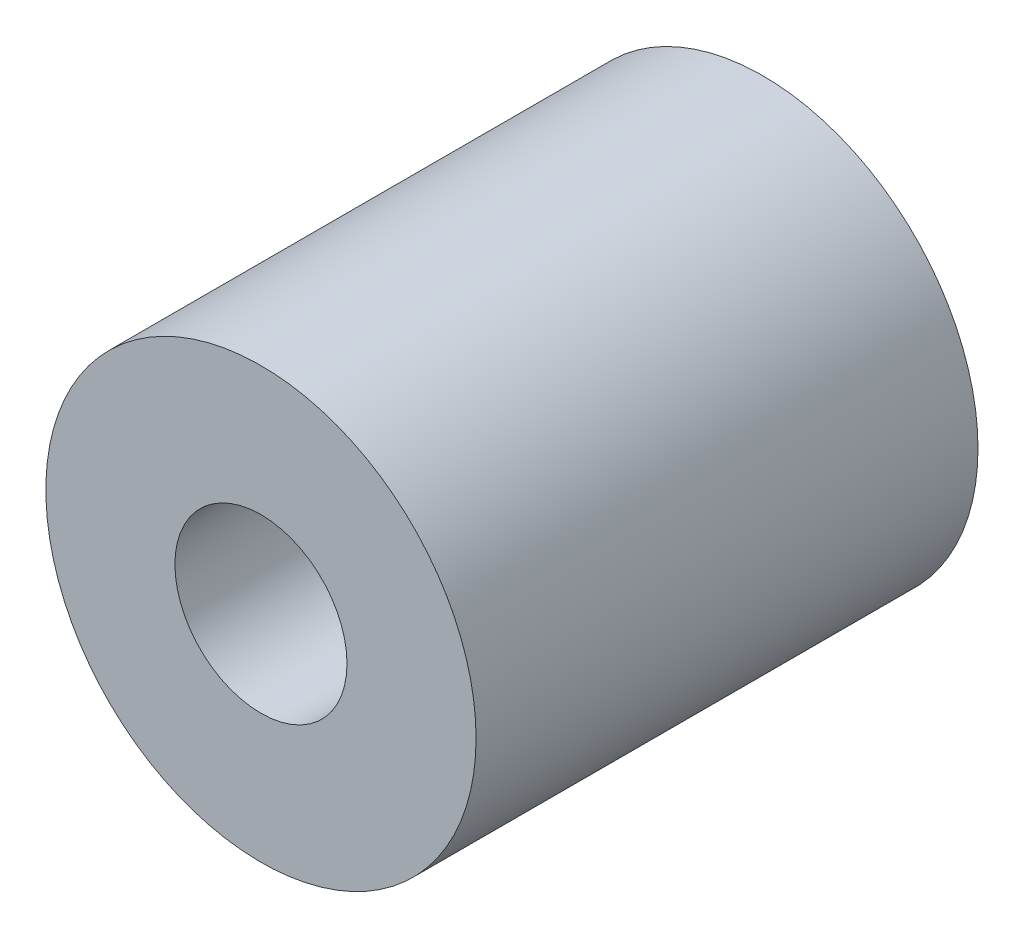
SolidWorks part; units mm, degrees
ref_plane "前视基准面" through (0, 0, 0) normal (0, 0, 1) x (1, 0, 0)
ref_plane "上视基准面" through (0, 0, 0) normal (0, 1, 0) x (1, 0, 0)
ref_plane "右视基准面" through (0, 0, 0) normal (1, 0, 0) x (0, 0, -1)
sketch "草图1" plane through (0, 0, 0) normal (0, 0, 1) x (1, 0, 0)
  circle A0 centre (0, 0) radius 15
  dimension "D1" = 30
extrude "凸台-拉伸1" add sketch "草图1" along normal blind 35
sketch "草图2" plane through (0, 0, 35) normal (0, 0, 1) x (1, 0, 0)
  circle A0 centre (0, 0) radius 6
  dimension "D1" = 12
extrude "切除-拉伸1" cut sketch "草图2" against normal blind 17.5
sketch "草图3" plane through (0, 0, 0) normal (0, 0, -1) x (-1, 0, 0)
  circle A0 centre (0, 0) radius 8
  dimension "D1" = 16
extrude "切除-拉伸2" cut sketch "草图3" against normal blind 17.5
